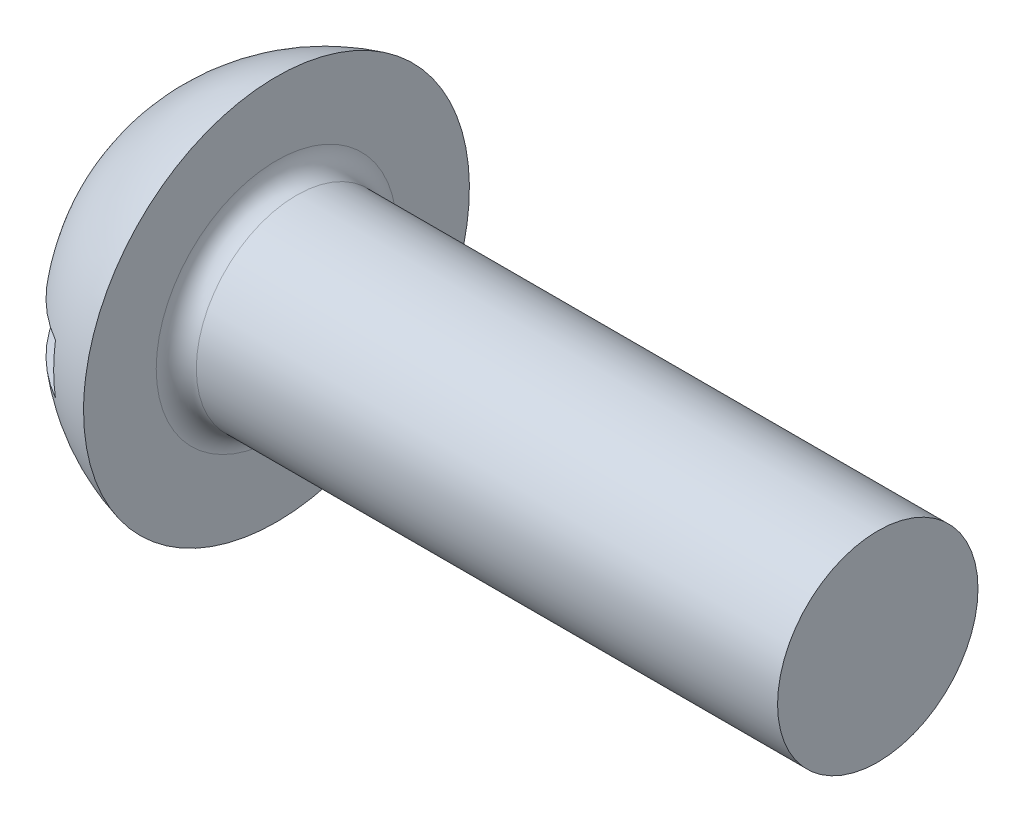
SolidWorks part; units mm, degrees
material "A2"
ref_plane "前视基准面" through (0, 0, 0) normal (0, 0, 1) x (1, 0, 0)
ref_plane "上视基准面" through (0, 0, 0) normal (0, 1, 0) x (1, 0, 0)
ref_plane "右视基准面" through (0, 0, 0) normal (1, 0, 0) x (0, 0, -1)
sketch "草图1" plane through (0, 0, 0) normal (0, 0, 1) x (1, 0, 0)
  line L0 (0, 0) -> (2, 0) construction
  line L1 (3, 3.85) -> (3, 2)
  line L2 (3, 2) -> (7, 2)
  line L3 (7, 2) -> (15, 2)
  line L4 (15, 2) -> (15, 0)
  line L5 (15, 0) -> (0, 0)
  line L6 (2, 0.5) -> (2, -0.5) construction
  line L7 (15, 0) -> (15.4, 0) construction
  arc A0 (0, 0) -> (3, 3.85) centre (3.9704, 0) cw
revolve "旋转1" add sketch "草图1" angle 360 about L0
cosmetic thread "装饰螺纹线1" parameters "D1"=8, "D2"=3.464
sketch "草图2" plane through (0, 0, 0) normal (1, 0, 0) x (0, 0, -1)
  line L0 (3.85, 0.5) -> (-3.85, 0.5)
  line L1 (-3.85, 0.5) -> (-3.85, -0.5)
  line L2 (-3.85, -0.5) -> (3.85, -0.5)
  line L3 (3.85, -0.5) -> (3.85, 0.5)
  circle A1 centre (0, 0) radius 3.85 construction
extrude "切除-拉伸1" cut sketch "草图2" along normal up to vertex (2 mm away) up to point (2, 0.5, 0)
fillet "圆角1" radius 0.4 1 edges at (3, 0, 2)
equation "\"D2@装饰螺纹线1\" = \"d@草图1\"*0.866"
equation "\"D1@装饰螺纹线1\" =\"l0@草图1\""
equation "\"D1@圆角1\" = \"r@草图1\""
